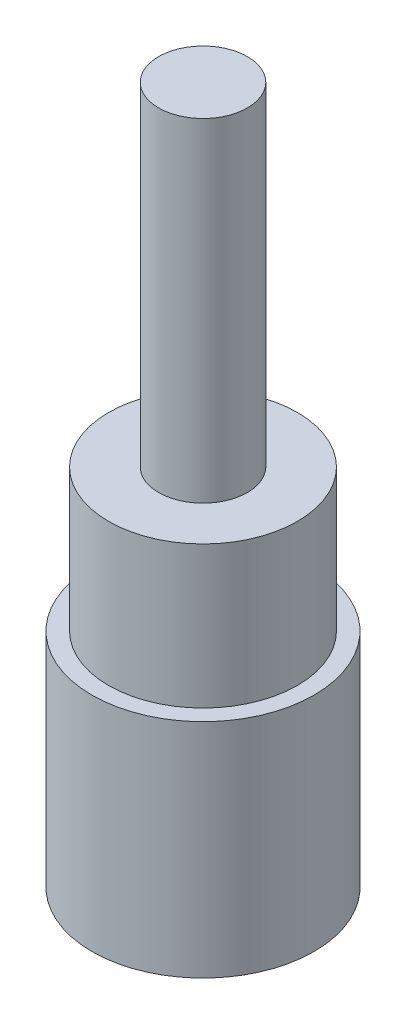
from build123d import *

# Parameters (mm, degrees)
SKETCH1_R           = 10
BOSS_EXTRUDE1_DEPTH = 20
SKETCH2_R           = 8.5
BOSS_EXTRUDE2_DEPTH = 12.8
SKETCH3_R           = 4
BOSS_EXTRUDE3_DEPTH = 30
CUT_EXTRUDE1_DEPTH  = 1.2


with BuildPart() as part:
    # Sketch1 → Boss-Extrude1 (new body)
    with BuildSketch(Plane(origin=(0, 0, 0), x_dir=(1, 0, 0), z_dir=(0, 1, 0))):
        with Locations(Location((0, 0, 0), (0, 0, 270))):
            Circle(SKETCH1_R)
    extrude(amount=BOSS_EXTRUDE1_DEPTH)

    # Sketch2 → Boss-Extrude2 (add)
    with BuildSketch(Plane(origin=(0, 20, 0), x_dir=(1, 0, 0), z_dir=(0, 1, 0))):
        with Locations(Location((0, 0, 0), (0, 0, 270))):
            Circle(SKETCH2_R)
    extrude(amount=BOSS_EXTRUDE2_DEPTH)

    # Sketch3 → Boss-Extrude3 (add)
    with BuildSketch(Plane(origin=(0, 32.8, 0), x_dir=(1, 0, 0), z_dir=(0, 1, 0))):
        with Locations(Location((0, 0, 0), (0, 0, 270))):
            Circle(SKETCH3_R)
    extrude(amount=BOSS_EXTRUDE3_DEPTH)

    # Sketch4 → Cut-Extrude1 (cut)
    with BuildSketch(Plane(origin=(0, 0, -4), x_dir=(-1, 0, 0), z_dir=(0, 0, -1))):
        with BuildLine():
            Line((1, 49.8), (1, 35.8))
            ThreePointArc((1, 35.8), (0, 34.8), (-1, 35.8))
            Line((-1, 35.8), (-1, 49.8))
            ThreePointArc((-1, 49.8), (0, 50.8), (1, 49.8))
        make_face()
    extrude(amount=-CUT_EXTRUDE1_DEPTH, mode=Mode.SUBTRACT)


solid = part.part
